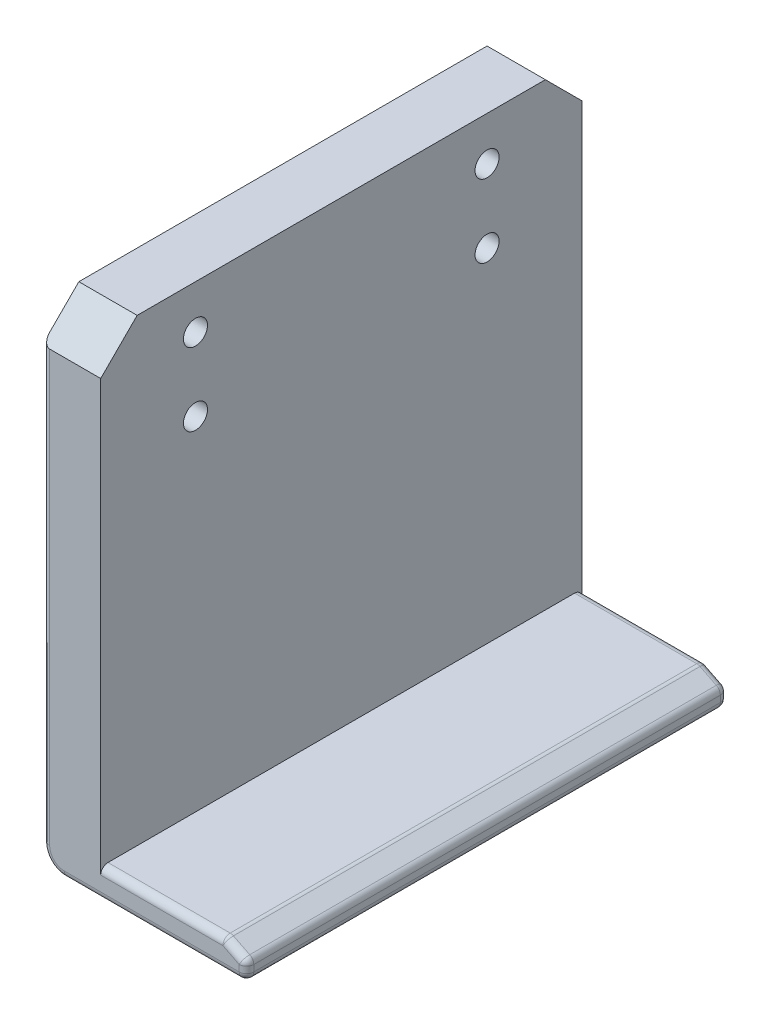
SolidWorks part; units mm, degrees
material "A6061"
ref_plane "前视基准面" through (0, 0, 0) normal (0, 0, 1) x (1, 0, 0)
ref_plane "上视基准面" through (0, 0, 0) normal (0, 1, 0) x (1, 0, 0)
ref_plane "右视基准面" through (0, 0, 0) normal (1, 0, 0) x (0, 0, -1)
sketch "草图1" plane through (0, 0, 0) normal (0, 0, 1) x (1, 0, 0)
  line L0 (0, 0) -> (0, 106.6965) construction
  line L1 (0, 67) -> (0, 0)
  line L2 (0, 0) -> (28, 0)
  line L3 (28, 0) -> (28, 4)
  line L4 (28, 4) -> (8, 4)
  line L5 (8, 4) -> (8, 67)
  line L6 (8, 67) -> (0, 67)
  dimension "D1" = 8
  dimension "D2" = 4
  dimension "D3" = 20
  dimension "D4" = 67
extrude "凸台-拉伸1" add sketch "草图1" along normal mid plane 66
chamfer "倒角1" distance 1.5 distance2 3 1 edges at (28, 4, 0)
fillet "圆角1" radius 1 3 edges at (28, 0, 0) (28, 2.5, 0) (25, 4, 0)
chamfer "倒角2" distance 5 angle 45 2 edges at (4, 67, 33) (4, 67, -33)
fillet "圆角3" radius 3 1 edges at (0, 0, 0)
fillet "圆角4" radius 1 18 edges at (0, 32.5, 33) (0.8787, 0.8787, 33) (15, 0, 33) (27.7071, 0.2929, 33) (28, 1.441, 33) (27.8507, 2.4077, 33) (26.3292, 3.3354, 33) (24.9937, 3.9732, 33) (0, 32.5, -33) (0.8787, 0.8787, -33) (15, 0, -33) (27.7071, 0.2929, -33) (28, 1.441, -33) (27.8507, 2.4077, -33) (26.3292, 3.3354, -33) (24.9937, 3.9732, -33) (16.382, 4, 33) (16.382, 4, -33)
hole_wizard "M4 螺纹孔2" positions "草图9" profile "草图8" tap size "M4" standard "GB" end condition through all
sketch "草图9" plane through (0, 0, 0) normal (-1, 0, 0) x (0, 0, 1)
  line L0 (0, 0) -> (0, 67) construction
  line L1 (28, 67) -> (-28, 67) construction
  point P0 (-20, 61)
  point P4 (20, 61)
  point P14 (-20, 51)
  point P16 (20, 51)
  dimension "D1" = 40
  dimension "D2" = 6
  dimension "D3" = 10
sketch "草图8" plane through (0, 61, -20) normal (0, 1, 0) x (0, 0, 1)
  line L0 (0, 0) -> (0, 28)
  line L1 (0, 28) -> (1.65, 28)
  line L2 (1.65, 28) -> (1.65, 0)
  line L5 (1.65, 0) -> (0, 0)
  line L11 (0, -6.35) -> (0, 107.95) construction
  dimension "通孔螺纹孔钻头直径" = 3.3
  dimension "通孔螺纹孔钻头深度" = 28
cosmetic thread "孔螺蚊线3" parameters "D2"=4
cosmetic thread "孔螺蚊线5" parameters "D2"=4
cosmetic thread "孔螺蚊线6" parameters "D2"=4
cosmetic thread "孔螺蚊线7" parameters "D2"=4
